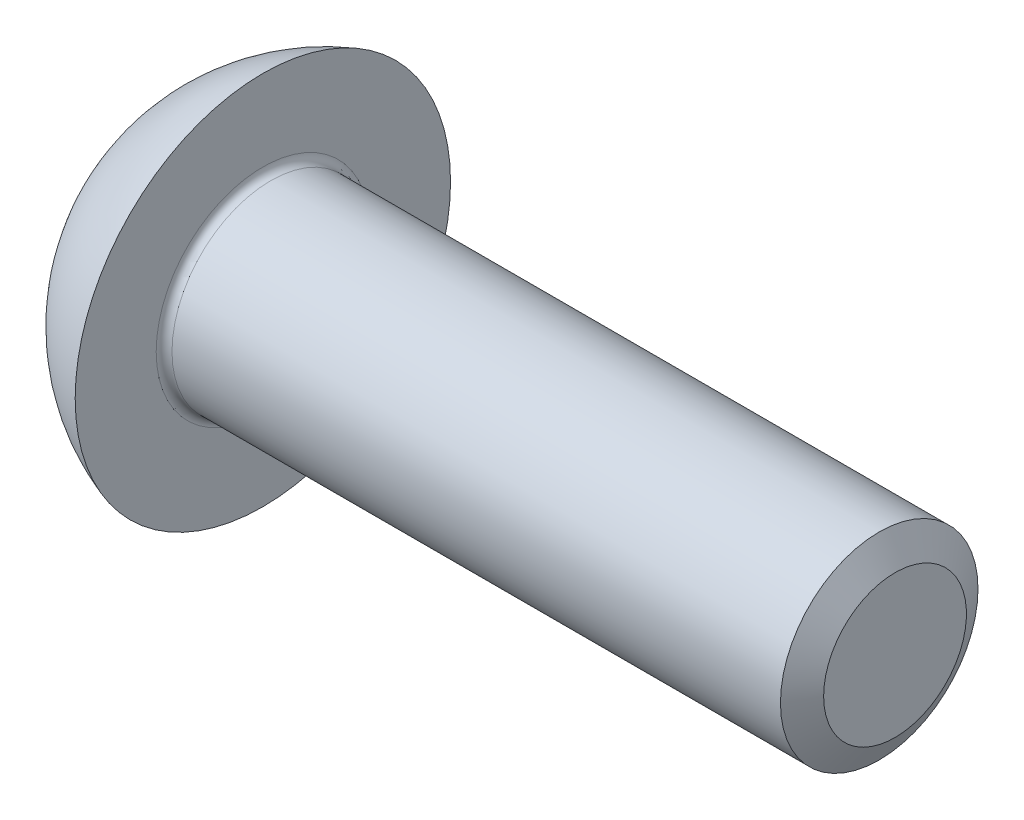
from build123d import *

# Parameters (mm, degrees)
CUT_EXTRUDE1_DEPTH = 2.75


with BuildPart() as part:
    # Sketch1 → Revolve1 (revolve)
    with BuildSketch(Plane.XY, mode=Mode.PRIVATE) as revolve1_sk:
        with BuildLine():
            Line((0, 2.5), (-15.8, 2.5))
            ThreePointArc((-15.8, 2.5), (-15.941421356, 2.558578644), (-16, 2.7))
            Line((-16, 2.7), (-16, 4.75))
            ThreePointArc((-16, 4.75), (-17.581194586, 3.877015605), (-18.75, 2.5))
            Line((-18.75, 2.5), (-18.75, 0))
            Line((-18.75, 0), (0, 0))
            Line((0, 0), (0, 2.5))
        make_face()
    revolve(revolve1_sk.sketch.rotate(Axis((-18.75, 0, 0), (1, 0, 0)), 90), axis=Axis((-18.75, 0, 0), (1, 0, 0)))

    # Sketch2 → Cut-Extrude1 (cut)
    with BuildSketch(Plane.ZY.offset(18.75)):
        Polygon((0, 1.732050808), (-1.5, 0.866025404), (-1.5, -0.866025404), (0, -1.732050808), (1.5, -0.866025404), (1.5, 0.866025404), align=None)
    extrude(amount=-CUT_EXTRUDE1_DEPTH, mode=Mode.SUBTRACT)

    # Sketch6 → Revolve2 (revolve)
    with BuildSketch(Plane.XY):
        Polygon((-17.19, 1.732050808), (-16, 0), (-15.56, 0), (-15.56, 1.732050808), align=None)
    revolve(axis=Axis((-18.75, 0, 0), (1, 0, 0)))

    # Sketch7 → Cut-Revolve5 (revolve, cut)
    with BuildSketch(Plane.XY):
        Polygon((-18.75, 1.732050808), (-18.31, 0), (-18.75, 0), align=None)
    revolve(axis=Axis((-18.75, 0, 0), (1, 0, 0)), mode=Mode.SUBTRACT)

    # Sketch4 → Cut-Revolve1 (revolve, cut)
    with BuildSketch(Plane.XY, mode=Mode.PRIVATE) as cut_revolve1_sk:
        Polygon((-0.4, 2.5), (0, 1.807179677), (0.4, 2.5), align=None)
    revolve(cut_revolve1_sk.sketch.rotate(Axis((-0.4, 0, 0), (1, 0, 0)), 90), axis=Axis((-0.4, 0, 0), (1, 0, 0)), mode=Mode.SUBTRACT)


solid = part.part
